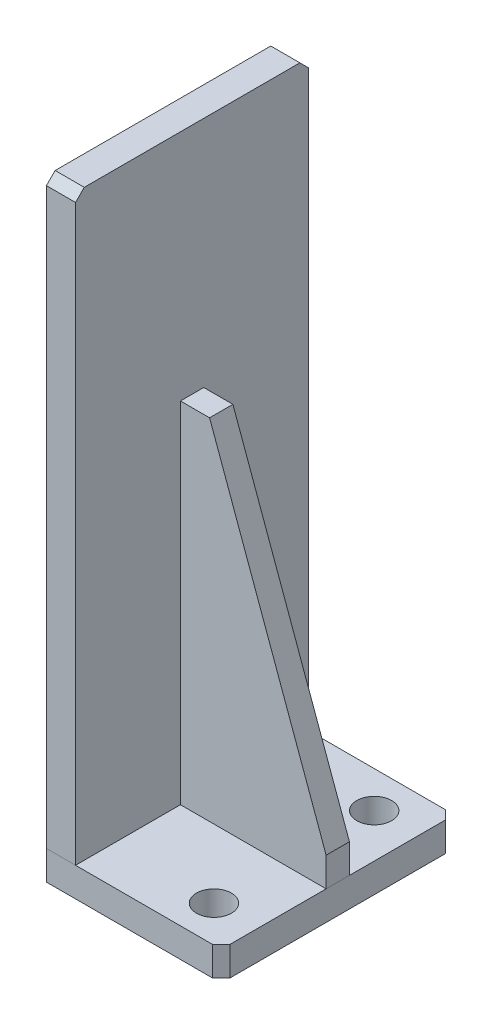
SolidWorks part; units mm, degrees
material "45#"
ref_plane "前基準面" through (0, 0, 0) normal (0, 0, 1) x (1, 0, 0)
ref_plane "上基準面" through (0, 0, 0) normal (0, 1, 0) x (1, 0, 0)
ref_plane "右基準面" through (0, 0, 0) normal (1, 0, 0) x (0, 0, -1)
sketch "草图1" plane through (0, 0, 0) normal (0, 1, 0) x (1, 0, 0)
  line L1 (-30, -40) -> (30, -40)
  line L2 (-30, -40) -> (-30, 40)
  line L3 (-30, 40) -> (30, 40)
  line L4 (30, -40) -> (30, 40)
  line L5 (-30, -40) -> (30, 40) construction
  line L6 (-30, 40) -> (30, -40) construction
  point P0 (0, 0)
  dimension "D1" = 60
  dimension "D2" = 80
extrude "凸台-拉伸1" add sketch "草图1" along normal mid plane 10
sketch "草图2" plane through (0, 5, 0) normal (0, 1, 0) x (1, 0, 0)
  line L0 (30, 40) -> (-30, 40) construction
  line L1 (-30, -40) -> (-20, -40)
  line L2 (-30, -40) -> (-30, 40)
  line L3 (-30, 40) -> (-20, 40)
  line L4 (-20, -40) -> (-20, 40)
  dimension "D1" = 10
extrude "凸台-拉伸2" add sketch "草图2" along normal blind 200 separate body
chamfer "倒角1" distance 3 angle 45 2 edges at (30, 0, -40) (30, 0, 40)
chamfer "倒角2" distance 3 angle 45 2 edges at (-25, 205, 40) (-25, 205, -40)
sketch "草图6" plane through (0, 0, 0) normal (0, 0, 1) x (1, 0, 0)
  line L0 (-20, 125) -> (-10, 125)
  line L1 (-20, 202) -> (-20, 5) construction
  line L2 (-10, 125) -> (30, 15)
  line L3 (30, 15) -> (30, 5)
  line L4 (30, 5) -> (-20, 5)
  line L5 (-20, 5) -> (-30, 5) construction
  line L6 (27, 5) -> (-30, 5) construction
  line L7 (-20, 5) -> (-20, 125)
  dimension "D1" = 10
  dimension "D2" = 120
extrude "凸台-拉伸3" add sketch "草图6" along normal mid plane 8 separate body
sketch "草图7" plane through (0, 5, 0) normal (0, 1, 0) x (1, 0, 0)
  line L0 (30, 0) -> (17.3303, 0) construction
  line L1 (30, -4) -> (30, 4) construction
  line L2 (30, -37) -> (30, 37) construction
  circle A0 centre (15, -27.5) radius 6
  circle A1 centre (15, 27.5) radius 6
  dimension "D1" = 12
  dimension "D2" = 55
  dimension "D3" = 15
extrude "切除-拉伸1" cut sketch "草图7" against normal blind 10
